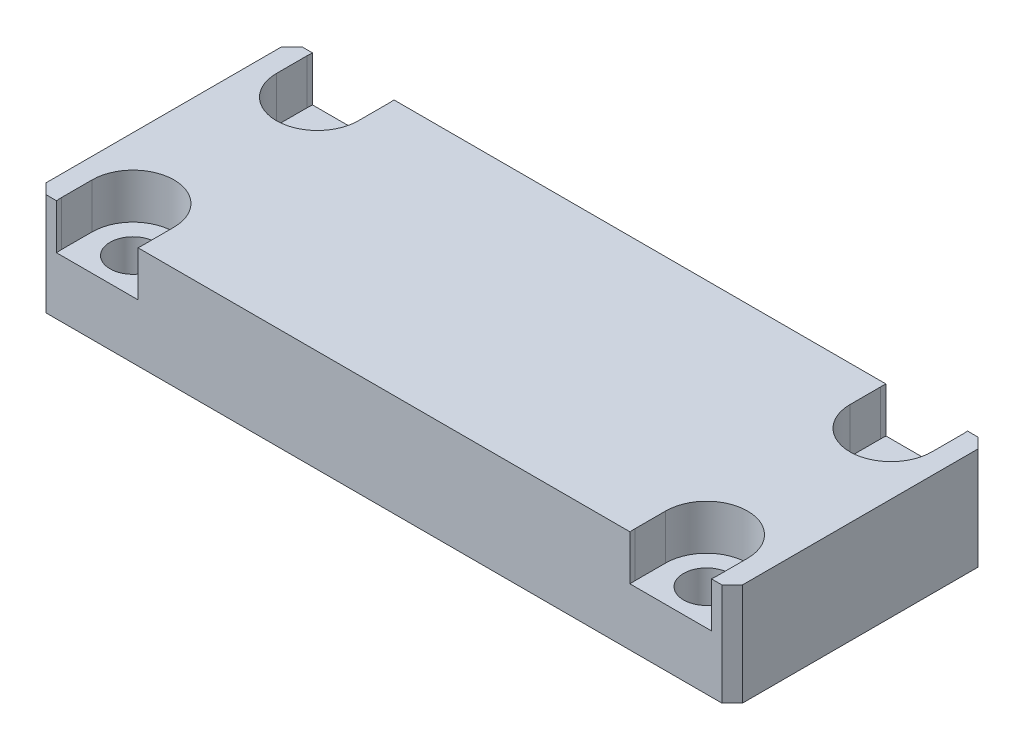
SolidWorks part; units mm, degrees
material "S45C"
ref_plane "前视基准面" through (0, 0, 0) normal (0, 0, 1) x (1, 0, 0)
ref_plane "上视基准面" through (0, 0, 0) normal (0, 1, 0) x (1, 0, 0)
ref_plane "右视基准面" through (0, 0, 0) normal (1, 0, 0) x (0, 0, -1)
sketch "草图1" plane through (0, 0, 0) normal (0, 1, 0) x (1, 0, 0)
  line L1 (-34, 12.5) -> (34, 12.5)
  line L2 (-34, 12.5) -> (-34, -12.5)
  line L3 (-34, -12.5) -> (34, -12.5)
  line L4 (34, 12.5) -> (34, -12.5)
  line L5 (-34, 12.5) -> (34, -12.5) construction
  line L6 (-34, -12.5) -> (34, 12.5) construction
  point P0 (0, 0)
  dimension "D1" = 68
  dimension "D2" = 25
extrude "凸台-拉伸1" add sketch "草图1" along normal mid plane 10
sketch "草图2" plane through (0, 5, 0) normal (0, 1, 0) x (1, 0, 0)
  line L0 (-28, 9) -> (28, 9) construction
  line L1 (28, 9) -> (28, -9) construction
  line L2 (28, -9) -> (-28, -9) construction
  line L3 (-28, -9) -> (-28, 9) construction
  line L5 (-28, 0) -> (0, 0) construction
  line L6 (0, 0) -> (0, 9) construction
  point P0 (-28, 9)
  point P3 (-28, -9)
  point P6 (28, 9)
  point P9 (28, -9)
  dimension "D1" = 56
  dimension "D2" = 18
hole_wizard "M4 六角凹头螺钉的柱形沉头孔1" positions "草图2" profile "草图3" counterbore size "M4" standard "ISO" end condition through all
sketch "草图3" plane through (-28, 5, -9) normal (1, 0, 0) x (0, 0, 1)
  line L0 (0, 0) -> (0, 10)
  line L1 (0, 10) -> (2.25, 10)
  line L3 (2.25, 10) -> (2.25, 4.4)
  line L4 (2.25, 4.4) -> (4, 4.4)
  line L5 (4, 4.4) -> (4, 0)
  line L7 (4, 0) -> (0, 0)
  line L11 (0, -6.35) -> (0, 107.95) construction
  dimension "通孔孔直径" = 4.5
  dimension "通孔孔深度" = 10
  dimension "柱形沉头孔直径" = 8
  dimension "柱形沉头孔深度" = 4.4
sketch "草图4" plane through (0, 5, 0) normal (0, 1, 0) x (1, 0, 0)
  line L0 (-28, 9) -> (-28, 12) construction
  line L1 (-32, 9) -> (-32, 12)
  line L2 (-24, 9) -> (-24, 12)
  line L3 (0, 0) -> (44.735, 0) construction
  line L4 (0, 0) -> (0, 23.5191) construction
  line L5 (-28, -9) -> (-28, -12) construction
  line L6 (-32, -9) -> (-32, -12)
  line L7 (-24, -9) -> (-24, -12)
  line L8 (28, 9) -> (28, 12) construction
  line L9 (32, 9) -> (32, 12)
  line L10 (24, 9) -> (24, 12)
  line L11 (28, -9) -> (28, -12) construction
  line L12 (32, -9) -> (32, -12)
  line L13 (24, -9) -> (24, -12)
  arc A0 (-32, 9) -> (-24, 9) centre (-28, 9) ccw
  arc A1 (-24, 12) -> (-32, 12) centre (-28, 12) ccw
  arc A2 (-29.9365, 12.5) -> (-26.0635, 12.5) centre (-28, 9) ccw construction
  arc A3 (-32, -9) -> (-24, -9) centre (-28, -9) cw
  arc A4 (-24, -12) -> (-32, -12) centre (-28, -12) cw
  arc A5 (32, 9) -> (24, 9) centre (28, 9) cw
  arc A6 (24, 12) -> (32, 12) centre (28, 12) cw
  arc A7 (32, -9) -> (24, -9) centre (28, -9) ccw
  arc A8 (24, -12) -> (32, -12) centre (28, -12) ccw
  point P3 (-28, 10.5)
  point P17 (-28, -10.5)
  point P24 (28, 10.5)
  point P31 (28, -10.5)
  dimension "D1" = 3
extrude "切除-拉伸1" cut sketch "草图4" against normal up to surface (4.4 mm away) up to face at (-28, 0.6, -6.75)
chamfer "倒角1" distance 1 angle 45 4 edges at (34, 0, -12.5) (34, 0, 12.5) (-34, 0, 12.5) (-34, 0, -12.5)
